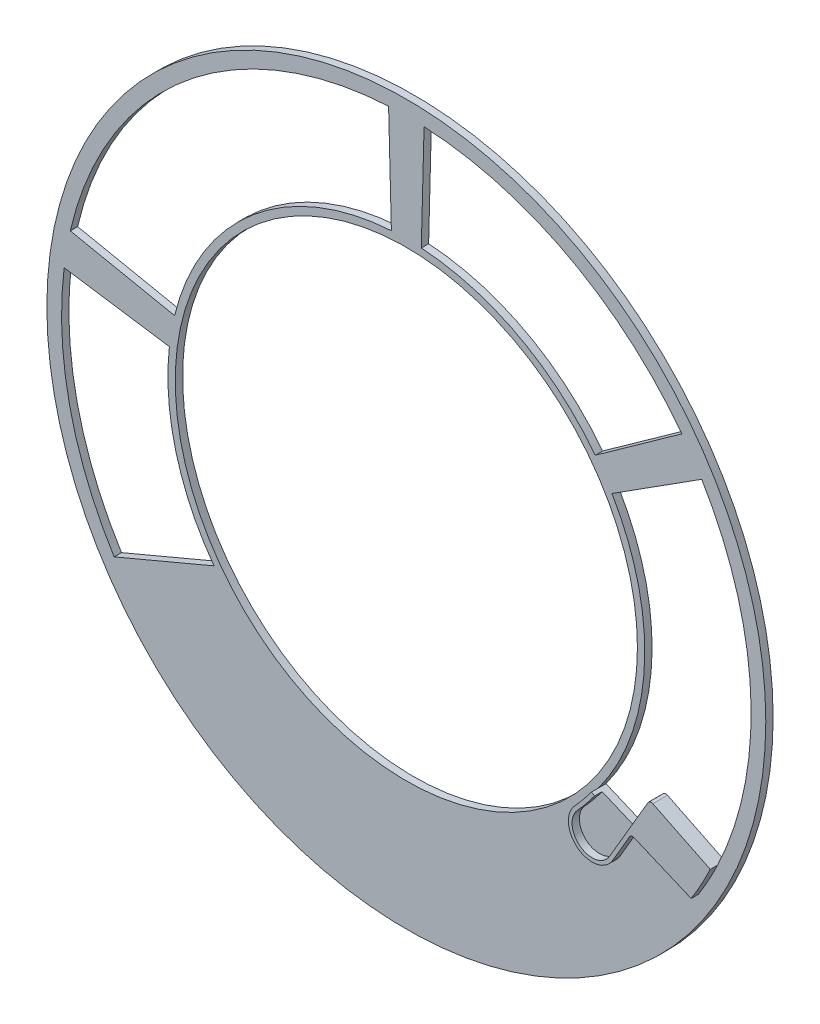
from build123d import *

# Parameters (mm, degrees)
SKETCH1_R           = 98
SKETCH1_R_2         = 63
BOSS_EXTRUDE1_DEPTH = 2
SKETCH2_R           = 94
SKETCH2_R_2         = 65
CUT_EXTRUDE2_DEPTH  = 5
BOSS_EXTRUDE2_DEPTH = 2
BOSS_EXTRUDE7_DEPTH = 2
BOSS_EXTRUDE9_DEPTH = 2
FILLET1_R           = 1


with BuildPart() as part:
    # Sketch1 → Boss-Extrude1 (new body)
    with BuildSketch(Plane.XY):
        Circle(SKETCH1_R)
        Circle(SKETCH1_R_2, mode=Mode.SUBTRACT)
    extrude(amount=BOSS_EXTRUDE1_DEPTH)

    # Sketch2 → Cut-Extrude2 (cut)
    with BuildSketch(Plane.XY.offset(2)):
        Circle(SKETCH2_R)
        Circle(SKETCH2_R_2, mode=Mode.SUBTRACT)
    extrude(amount=-CUT_EXTRUDE2_DEPTH, mode=Mode.SUBTRACT)


with BuildPart() as cut_extrude2_piece_1:
    # of the separate pieces the step leaves, piece 1, a body of its own (cut_extrude2_pieces)
    add(part.part.solids().sort_by_distance((98, 0, 0))[0])



with BuildPart() as cut_extrude2_piece_2:
    # of the separate pieces the step leaves, piece 2, a body of its own (cut_extrude2_pieces)
    add(part.part.solids().sort_by_distance((65, 0, 0))[0])


with BuildPart() as cut_extrude2_piece_1_1:
    add(cut_extrude2_piece_1.part)

    add(cut_extrude2_piece_2.part)  # Boss-Extrude2 merges Cut-Extrude2 piece 2
    # Sketch3 → Boss-Extrude2 (add)
    with BuildSketch(Plane.XY.offset(2)):
        with BuildLine():
            Line((4.836242993, 93.875506676), (4.076760177, 64.872028074))
            ThreePointArc((4.076760177, 64.872028074), (0, 65), (-4.076760177, 64.872028074))
            Line((-4.076760177, 64.872028074), (-4.836242993, 93.875506676))
            ThreePointArc((-4.836242993, 93.875506676), (0, 94), (4.836242993, 93.875506676))
        make_face()
        with BuildLine():
            Line((75.121929416, 56.503944294), (51.501653321, 39.655765094))
            ThreePointArc((51.501653321, 39.655765094), (53.887442216, 36.347538726), (56.061044042, 32.896190372))
            Line((56.061044042, 32.896190372), (80.530714938, 48.485089992))
            ThreePointArc((80.530714938, 48.485089992), (77.92953182, 52.564132926), (75.121929416, 56.503944294))
        make_face()
        with BuildLine():
            Line((-93.289131575, 11.538541067), (-64.594398177, 7.250084427))
            ThreePointArc((-64.594398177, 7.250084427), (-64.012503946, 11.287131548), (-63.178554226, 15.279734486))
            Line((-63.178554226, 15.279734486), (-91.60952201, 21.064080257))
            ThreePointArc((-91.60952201, 21.064080257), (-92.571928783, 16.322928701), (-93.289131575, 11.538541067))
        make_face()
    extrude(amount=-BOSS_EXTRUDE2_DEPTH)

    # Sketch8 → Boss-Extrude7 (add)
    with BuildSketch(Plane.XY.offset(2)):
        with BuildLine():
            Line((-52.42405813, -38.428090366), (-79.6500328, -49.918656582))
            ThreePointArc((-79.6500328, -49.918656582), (0, -94), (79.6500328, -49.918656582))
            Line((79.6500328, -49.918656582), (52.42405813, -38.428090366))
            ThreePointArc((52.42405813, -38.428090366), (0, -65), (-52.42405813, -38.428090366))
        make_face()
    extrude(amount=-BOSS_EXTRUDE7_DEPTH)

    # Sketch9 → Boss-Extrude9 (add, symmetric)
    with BuildSketch(Plane.XY.offset(2)):
        with BuildLine():
            Line((68.281233408, -34.472640013), (63.286378857, -43.012470433))
            Line((63.286378857, -43.012470433), (79.6500328, -49.918656582))
            ThreePointArc((79.6500328, -49.918656582), (82.146531581, -45.694062516), (84.419166177, -41.344943851))
            Line((84.419166177, -41.344943851), (69.584267033, -34.079436503))
            ThreePointArc((69.584267033, -34.079436503), (68.855533807, -34.020151468), (68.281233408, -34.472640013))
        make_face()
        with BuildLine():
            Line((67.88695627, -33.166048499), (62.357246072, -42.620335278))
            Line((62.357246072, -42.620335278), (63.286378857, -43.012470433))
            Line((63.286378857, -43.012470433), (68.281233408, -34.472640013))
            ThreePointArc((68.281233408, -34.472640013), (68.855533807, -34.020151468), (69.584267033, -34.079436503))
            Line((69.584267033, -34.079436503), (84.419166177, -41.344943851))
            ThreePointArc((84.419166177, -41.344943851), (84.63789491, -40.895314466), (84.854228869, -40.444527975))
            Line((84.854228869, -40.444527975), (69.189989894, -32.772844989))
            ThreePointArc((69.189989894, -32.772844989), (68.461256668, -32.713559953), (67.88695627, -33.166048499))
        make_face()
        with BuildLine():
            Line((62.357246072, -42.620335278), (57.396762094, -51.10140145))
            ThreePointArc((57.396762094, -51.10140145), (49.408790851, -52.744247062), (48.625615223, -44.626780572))
            ThreePointArc((48.625615223, -44.626780572), (51.08046785, -41.794566683), (53.370590226, -38.8275688))
            Line((53.370590226, -38.8275688), (52.42405813, -38.428090366))
            ThreePointArc((52.42405813, -38.428090366), (50.232411211, -41.251725587), (47.888863477, -43.95061723))
            ThreePointArc((47.888863477, -43.95061723), (48.814898229, -53.548791376), (58.259955891, -51.606274177))
            Line((58.259955891, -51.606274177), (63.286378857, -43.012470433))
            Line((63.286378857, -43.012470433), (62.357246072, -42.620335278))
        make_face()
    extrude(amount=BOSS_EXTRUDE9_DEPTH, both=True)

    # Fillet1
    fillet1_edges = [cut_extrude2_piece_1_1.edges().sort_by_distance(p)[0] for p in [
        (63.286378857, -43.012470433, 3),
    ]]
    fillet(fillet1_edges, radius=FILLET1_R)


solid = cut_extrude2_piece_1_1.part
